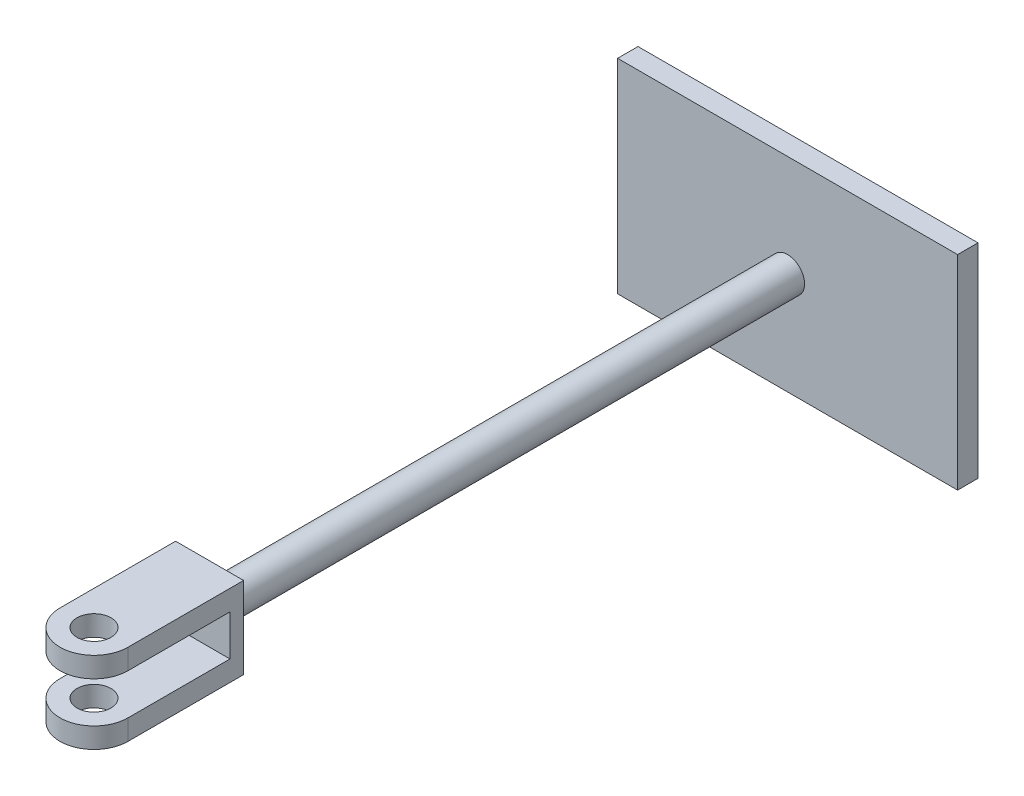
SolidWorks part; units mm, degrees
ref_plane "Front Plane" through (0, 0, 0) normal (0, 0, 1) x (1, 0, 0)
ref_plane "Top Plane" through (0, 0, 0) normal (0, 1, 0) x (1, 0, 0)
ref_plane "Right Plane" through (0, 0, 0) normal (1, 0, 0) x (0, 0, -1)
other "Configuration Table"
sketch "Sketch1" plane through (0, 0, 0) normal (0, 0, 1) x (1, 0, 0)
  line L1 (-25, 15) -> (25, 15)
  line L2 (-25, 15) -> (-25, -15)
  line L3 (-25, -15) -> (25, -15)
  line L4 (25, 15) -> (25, -15)
  line L5 (-25, 15) -> (25, -15) construction
  line L6 (-25, -15) -> (25, 15) construction
  point P0 (0, 0)
  dimension "D1" = 50
  dimension "D2" = 30
extrude "Boss-Extrude1" add sketch "Sketch1" along normal blind 3
sketch "Sketch2" plane through (0, 0, 3) normal (0, 0, 1) x (1, 0, 0)
  circle A0 centre (0, 0) radius 2.5
  dimension "D1" = 5
extrude "Boss-Extrude2" add sketch "Sketch2" along normal blind 85
sketch "Sketch3" plane through (0, 0, 88) normal (0, 0, 1) x (1, 0, 0)
  line L1 (-5, 6) -> (5, 6)
  line L2 (-5, 6) -> (-5, -6)
  line L3 (-5, -6) -> (5, -6)
  line L4 (5, 6) -> (5, -6)
  line L5 (-5, 6) -> (5, -6) construction
  line L6 (-5, -6) -> (5, 6) construction
  point P0 (0, 0)
  dimension "D1" = 10
  dimension "D2" = 12
extrude "Boss-Extrude3" add sketch "Sketch3" along normal blind 22
sketch "Sketch4" plane through (0, 0, 110) normal (0, 0, 1) x (1, 0, 0)
  line L1 (-8.7981, 3) -> (8.7981, 3)
  line L2 (-8.7981, 3) -> (-8.7981, -3)
  line L3 (-8.7981, -3) -> (8.7981, -3)
  line L4 (8.7981, 3) -> (8.7981, -3)
  line L5 (-8.7981, 3) -> (8.7981, -3) construction
  line L6 (-8.7981, -3) -> (8.7981, 3) construction
  point P0 (0, 0)
  dimension "D1" = 6
extrude "Cut-Extrude1" cut sketch "Sketch4" against normal blind 20
sketch "Sketch5" plane through (0, -6, 0) normal (0, -1, 0) x (-1, 0, 0)
  line L0 (5, -110) -> (-5, -110) construction
  line L1 (5, -105) -> (16.8654, -140.3256)
  line L2 (16.8654, -140.3256) -> (-16.12, -140.3256)
  line L3 (-16.12, -140.3256) -> (-5, -105)
  circle A0 centre (0, -105) radius 2.5
  arc A1 (-5, -105) -> (5, -105) centre (0, -105) ccw
  dimension "D1" = 5
  dimension "D2" = 5
extrude "Cut-Extrude2" cut sketch "Sketch5" against normal through all
